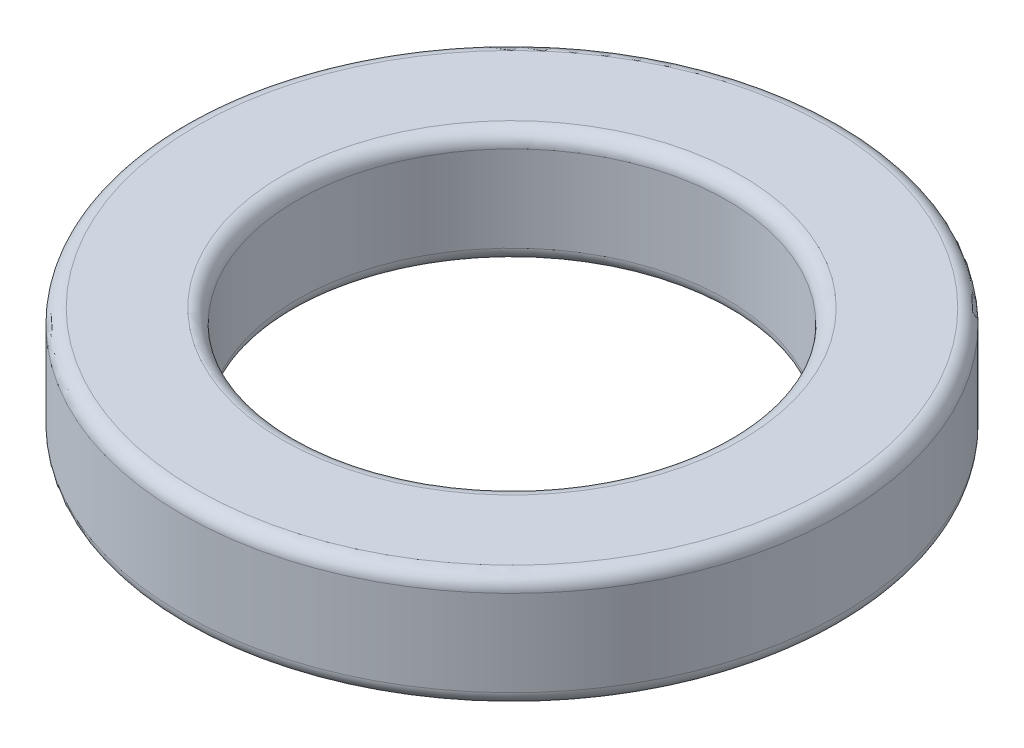
from build123d import *

# Parameters (mm, degrees)
SKETCH_1_R      = 2.3
SKETCH_1_R_2    = 1.5
EXTRUDE_1_DEPTH = 0.8
FILLET_1_R      = 0.1


with BuildPart() as part:
    # 草图1 → 凸台-拉伸1 (new body)
    with BuildSketch(Plane(origin=(0, 0, 0), x_dir=(1, 0, 0), z_dir=(0, 1, 0))):
        with Locations(Location((0, 0, 0), (0, 0, 270))):
            Circle(SKETCH_1_R)
        with Locations(Location((0, 0, 0), (0, 0, 270))):
            Circle(SKETCH_1_R_2, mode=Mode.SUBTRACT)
    extrude(amount=EXTRUDE_1_DEPTH)

    # 圆角1
    fillet_1_edges = [part.edges().sort_by_distance(p)[0] for p in [
        (0, 0, -2.3),
        (0, 0.8, -2.3),
        (0, 0, -1.5),
        (0, 0.8, -1.5),
    ]]
    fillet(fillet_1_edges, radius=FILLET_1_R)


solid = part.part
